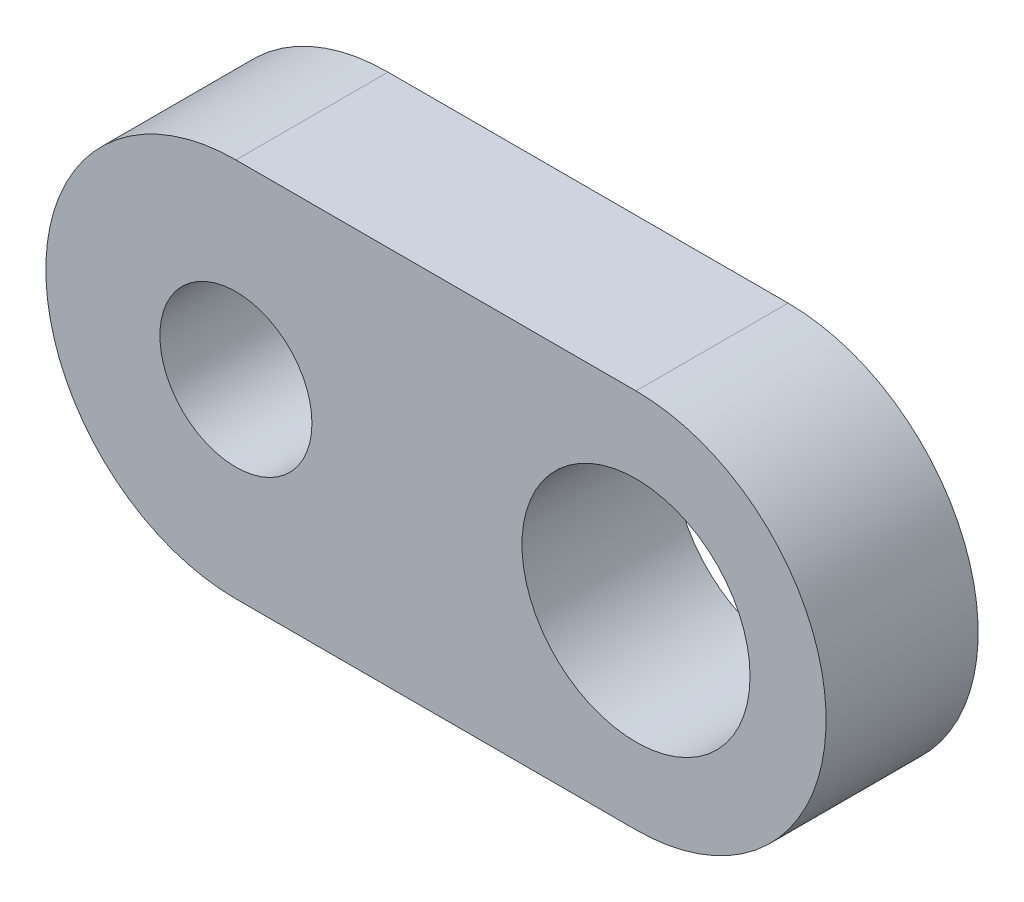
from build123d import *

# Parameters (mm, degrees)
SKETCH_1_R      = 7.5
SKETCH_1_R_2    = 5
EXTRUDE_1_DEPTH = 10


with BuildPart() as part:
    # 草图1 → 凸台-拉伸1 (new body)
    with BuildSketch(Plane.XY):
        with BuildLine():
            Line((-13.155, 12.5), (13.155, 12.5))
            ThreePointArc((13.155, 12.5), (25.655, 0), (13.155, -12.5))
            Line((13.155, -12.5), (-13.155, -12.5))
            ThreePointArc((-13.155, -12.5), (-25.655, 0), (-13.155, 12.5))
        make_face()
        with Locations((13.155, 0)):
            Circle(SKETCH_1_R, mode=Mode.SUBTRACT)
        with Locations((-13.155, 0)):
            Circle(SKETCH_1_R_2, mode=Mode.SUBTRACT)
    extrude(amount=EXTRUDE_1_DEPTH)


solid = part.part
